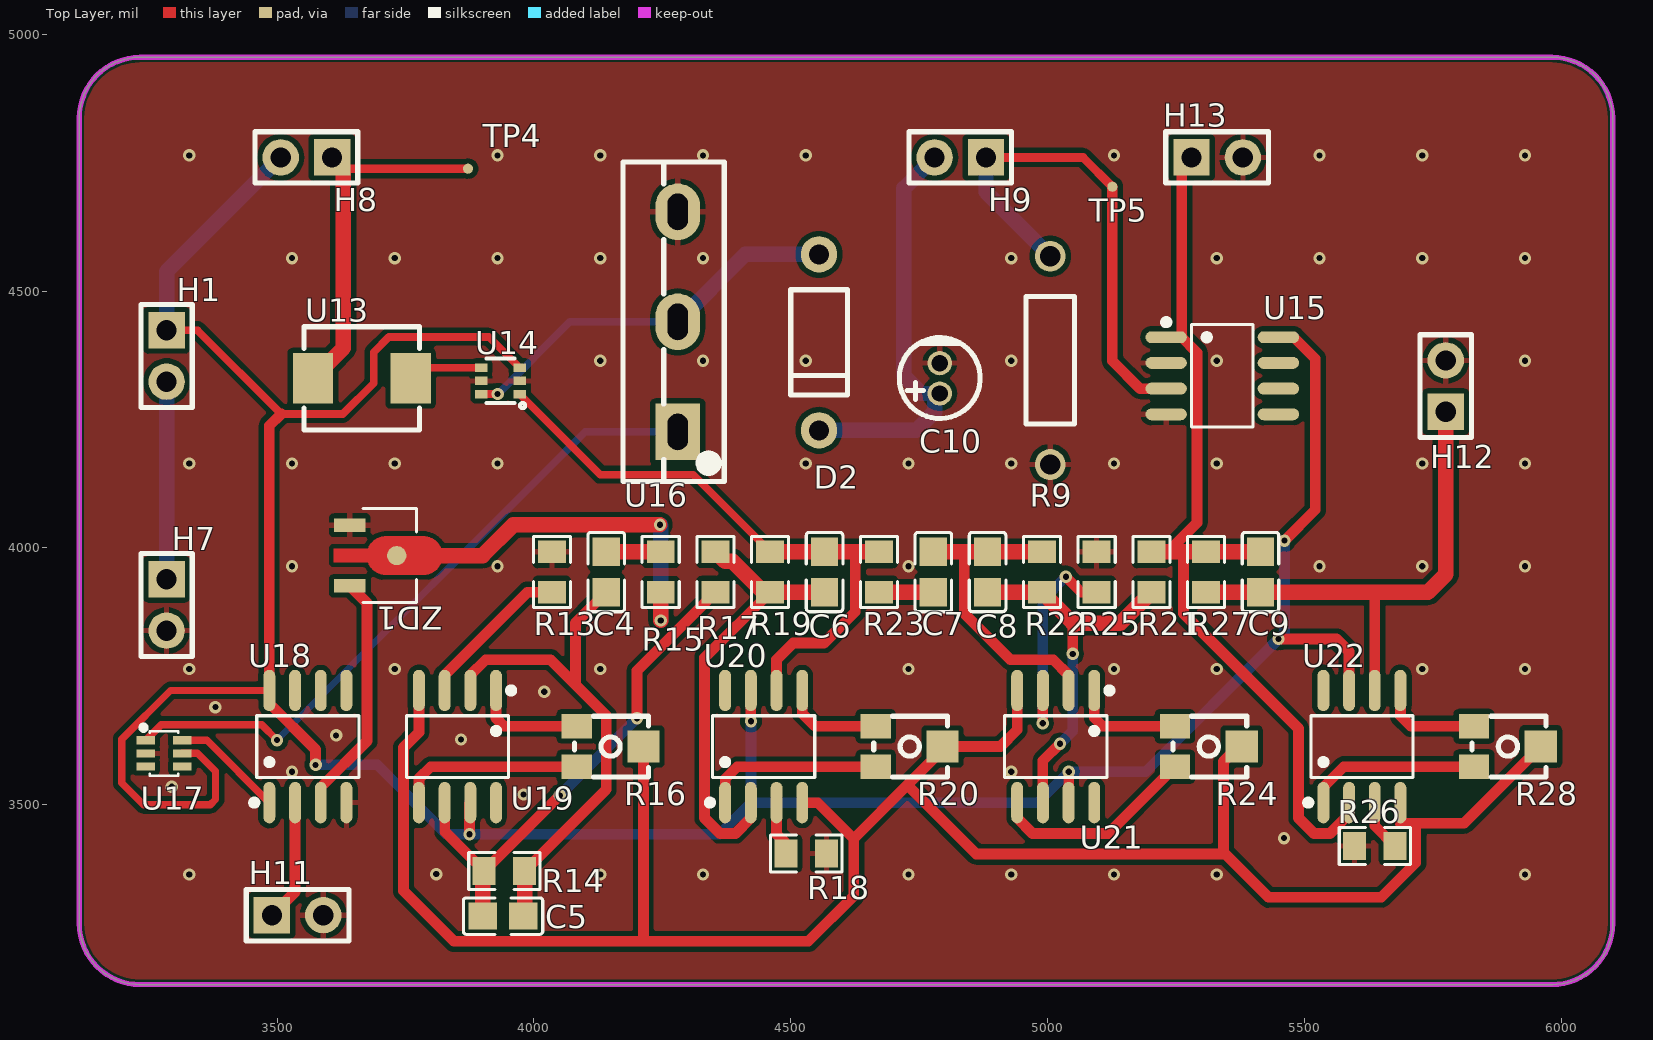
[diagram p0: Top Layer view]
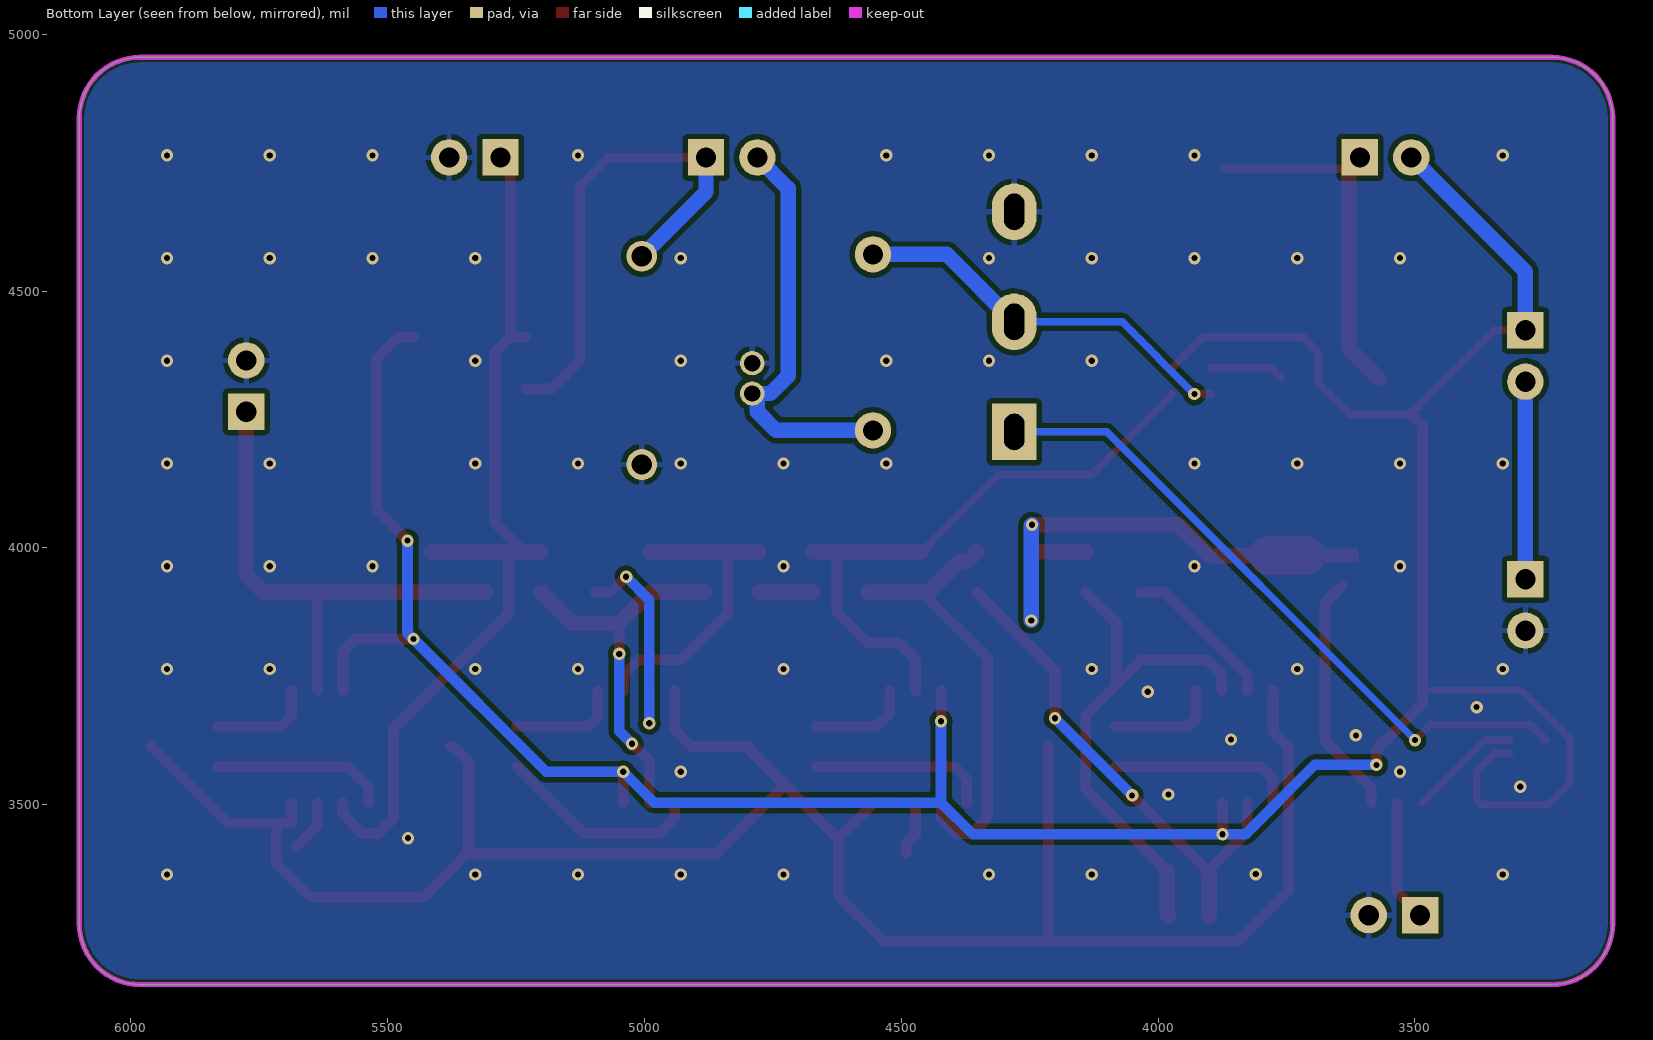
[diagram p1: Bottom Layer view, seen from below]
# Altium PCB MISC52076.pcbdoc
Units mil, origin at the board's own origin, x right, y up, seen from the top; angles counter-clockwise.
Board outline 2985 x 1805 mil, 2 copper layers (Top Layer, Bottom Layer), stack 62.206 mil thick; 45 components, 36 nets, 138 pads, 84 vias.

## Layer stack, top to bottom
Top Solder Mask Layer: solder mask 0.394, Dk 3.3
Top Layer: signal copper 1.379
Dielectric1: surface 59.449, FR4, Dk 4.5
Bottom Layer: signal copper 1.378
Bottom Solder Mask Layer: solder mask 0.394, Dk 3.3

## Board outline
3233.11,4955 ccw(c3233.11,4836.89) 3115,4836.89 3115,3268.11 ccw(c3233.11,3268.11) 3233.11,3150 5981.89,3150 ccw(c5981.89,3268.11) 6100,3268.11 6100,4836.89 ccw(c5981.89,4836.89) 5981.89,4955

## Design rules (kind name [scope] priority, off if disabled: settings)
BoardOutlineClearance copperThickness2oz_1 [All] p2 off: genericclearance=7.99 ignorepadtopadclearanceinfootprint=FALSE except(0: Arc-SplitContinuation Track-SplitContinuation SMDPad-SplitContinuation THPad-SplitContinuation Via-SplitContinuation Fill-SplitContinuation Region-SplitContinuation Poly-SplitContinuation Text-SplitContinuation Hole-SplitContinuation; 5.98: Arc-CutoutEdge Track-CutoutEdge SMDPad-CutoutEdge THPad-CutoutEdge Via-CutoutEdge Text-CutoutEdge; 6.89: Hole-OutlineEdge Hole-CutoutEdge; 10: Poly-OutlineEdge Poly-CutoutEdge; 11.81: Arc-OutlineEdge Track-OutlineEdge SMDPad-OutlineEdge THPad-OutlineEdge Via-OutlineEdge Fill-OutlineEdge Region-OutlineEdge Text-OutlineEdge Fill-CutoutEdge Region-CutoutEdge)
BoardOutlineClearance Plane_innerPlane_1 [All] p4 off: genericclearance=4.02 ignorepadtopadclearanceinfootprint=FALSE except(0: Arc-SplitContinuation Track-SplitContinuation SMDPad-SplitContinuation THPad-SplitContinuation Via-SplitContinuation Fill-SplitContinuation Region-SplitContinuation Poly-SplitContinuation Text-SplitContinuation Hole-SplitContinuation; 5.98: Arc-CutoutEdge Track-CutoutEdge SMDPad-CutoutEdge THPad-CutoutEdge Via-CutoutEdge Text-CutoutEdge; 6.89: Hole-OutlineEdge Hole-CutoutEdge; 10: Poly-OutlineEdge Poly-CutoutEdge; 11.81: Arc-OutlineEdge Track-OutlineEdge SMDPad-OutlineEdge THPad-OutlineEdge Via-OutlineEdge Fill-OutlineEdge Region-OutlineEdge Text-OutlineEdge Fill-CutoutEdge Region-CutoutEdge)
BoardOutlineClearance Copper_copperRegion_1 [All] p6 off: genericclearance=4.02 ignorepadtopadclearanceinfootprint=FALSE except(0: Arc-SplitContinuation Track-SplitContinuation SMDPad-SplitContinuation THPad-SplitContinuation Via-SplitContinuation Fill-SplitContinuation Region-SplitContinuation Poly-SplitContinuation Text-SplitContinuation Hole-SplitContinuation; 5.98: Arc-CutoutEdge Track-CutoutEdge SMDPad-CutoutEdge THPad-CutoutEdge Via-CutoutEdge Text-CutoutEdge; 6.89: Hole-OutlineEdge Hole-CutoutEdge; 10: Poly-OutlineEdge Poly-CutoutEdge; 11.81: Arc-OutlineEdge Track-OutlineEdge SMDPad-OutlineEdge THPad-OutlineEdge Via-OutlineEdge Fill-OutlineEdge Region-OutlineEdge Text-OutlineEdge Fill-CutoutEdge Region-CutoutEdge)
BoardOutlineClearance copperThickness1oz_1 [All] p8: genericclearance=4.02 ignorepadtopadclearanceinfootprint=FALSE except(0: Arc-SplitContinuation Track-SplitContinuation SMDPad-SplitContinuation THPad-SplitContinuation Via-SplitContinuation Fill-SplitContinuation Region-SplitContinuation Poly-SplitContinuation Text-SplitContinuation Hole-SplitContinuation; 5.98: Arc-CutoutEdge Track-CutoutEdge SMDPad-CutoutEdge THPad-CutoutEdge Via-CutoutEdge Text-CutoutEdge; 6.89: Hole-OutlineEdge Hole-CutoutEdge; 10: Poly-OutlineEdge Poly-CutoutEdge; 11.81: Arc-OutlineEdge Track-OutlineEdge SMDPad-OutlineEdge THPad-OutlineEdge Via-OutlineEdge Fill-OutlineEdge Region-OutlineEdge Text-OutlineEdge Fill-CutoutEdge Region-CutoutEdge)
Clearance copperThickness2oz [All] p1 off: gap=7.99 ignorepadtopadclearanceinfootprint=FALSE except(5.98: SMDPad-Track SMDPad-SMDPad THPad-Track SMDPad-THPad THPad-THPad Track-Via SMDPad-Via THPad-Via Via-Via Fill-SMDPad Region-SMDPad Fill-THPad Region-THPad Fill-Via Region-Via Fill-Fill Fill-Region Region-Region Arc-Track Arc-SMDPad Arc-THPad Arc-Via Fill-Arc Region-Arc Arc-Arc Text-Track SMDPad-Text Text-THPad Text-Via Fill-Text Region-Text Arc-Text Text-Text; 6.89: Hole-Track Hole-SMDPad Hole-THPad Hole-Via Fill-Hole Region-Hole Hole-Arc Hole-Text; 10: Poly-Track Poly-SMDPad Poly-THPad Poly-Via Poly-Fill Poly-Region Poly-Poly Poly-Arc Poly-Text Poly-Hole; 11.81: Fill-Track Region-Track)
Clearance Plane_innerPlane [All] p3 off: gap=4.02 ignorepadtopadclearanceinfootprint=FALSE except(5.98: SMDPad-Track SMDPad-SMDPad THPad-Track SMDPad-THPad THPad-THPad Track-Via SMDPad-Via THPad-Via Via-Via Fill-SMDPad Region-SMDPad Fill-THPad Region-THPad Fill-Via Region-Via Fill-Fill Fill-Region Region-Region Arc-Track Arc-SMDPad Arc-THPad Arc-Via Fill-Arc Region-Arc Arc-Arc Text-Track SMDPad-Text Text-THPad Text-Via Fill-Text Region-Text Arc-Text Text-Text; 6.89: Hole-Track Hole-SMDPad Hole-THPad Hole-Via Fill-Hole Region-Hole Hole-Arc Hole-Text; 10: Poly-Track Poly-SMDPad Poly-THPad Poly-Via Poly-Fill Poly-Region Poly-Poly Poly-Arc Poly-Text Poly-Hole; 11.81: Fill-Track Region-Track)
Clearance Copper_copperRegion [All] p5 off: gap=4.02 ignorepadtopadclearanceinfootprint=FALSE except(5.98: SMDPad-Track SMDPad-SMDPad THPad-Track SMDPad-THPad THPad-THPad Track-Via SMDPad-Via THPad-Via Via-Via Fill-SMDPad Region-SMDPad Fill-THPad Region-THPad Fill-Via Region-Via Fill-Fill Fill-Region Region-Region Arc-Track Arc-SMDPad Arc-THPad Arc-Via Fill-Arc Region-Arc Arc-Arc Text-Track SMDPad-Text Text-THPad Text-Via Fill-Text Region-Text Arc-Text Text-Text; 6.89: Hole-Track Hole-SMDPad Hole-THPad Hole-Via Fill-Hole Region-Hole Hole-Arc Hole-Text; 10: Poly-Track Poly-SMDPad Poly-THPad Poly-Via Poly-Fill Poly-Region Poly-Poly Poly-Arc Poly-Text Poly-Hole; 11.81: Fill-Track Region-Track)
Clearance copperThickness1oz [All] p7: gap=4.02 ignorepadtopadclearanceinfootprint=FALSE except(5.98: SMDPad-Track SMDPad-SMDPad THPad-Track SMDPad-THPad THPad-THPad Track-Via SMDPad-Via THPad-Via Via-Via Fill-SMDPad Region-SMDPad Fill-THPad Region-THPad Fill-Via Region-Via Fill-Fill Fill-Region Region-Region Arc-Track Arc-SMDPad Arc-THPad Arc-Via Fill-Arc Region-Arc Arc-Arc Text-Track SMDPad-Text Text-THPad Text-Via Fill-Text Region-Text Arc-Text Text-Text; 6.89: Hole-Track Hole-SMDPad Hole-THPad Hole-Via Fill-Hole Region-Hole Hole-Arc Hole-Text; 10: Poly-Track Poly-SMDPad Poly-THPad Poly-Via Poly-Fill Poly-Region Poly-Poly Poly-Arc Poly-Text Poly-Hole; 11.81: Fill-Track Region-Track)
DiffPairsRouting differentialPair [All] p1: maxlimit=6 minlimit=6 mostfreqgap=6 toplayer_minwidth=5 toplayer_prefwidth=10 toplayer_maxwidth=100 toplayer_mingap=6 toplayer_prefgap=6 toplayer_maxgap=6 bottomlayer_minwidth=5 bottomlayer_prefwidth=10 bottomlayer_maxwidth=100 bottomlayer_mingap=6 bottomlayer_prefgap=6 bottomlayer_maxgap=6 maxuncoupledlength=10
HoleToHoleClearance otherClearance [All] p1: gap=11.81 allowstackedmicrovias=TRUE
Length netLength [All] p1: minlimit=0 maxlimit=0
PasteMaskExpansion pasteMaskExpansion [All] p1: expansion=0
PlaneConnect innerPlane [All] p1: planeconnectstyle=Relief reliefexpansion=20 reliefentries=4 reliefconductorwidth=10 reliefairgap=10
PolygonConnect copperRegion [All] p1: connectstyle=Relief reliefconductorwidth=10 reliefentries=4 polygonreliefangle="90 Angle" airgapwidth=10 via.connectstyle=Relief via.reliefconductorwidth=10 via.reliefentries=4 via.polygonreliefangle="90 Angle" via.airgapwidth=10
RoutingVias viaSize [All] p1: holewidth=12.01 width=24.02 viastyle="Through Hole" minholewidth=11.81 minwidth=19.68 maxholewidth=248.03 maxwidth=393.7
SolderMaskExpansion solderMaskExpansion [IsVia] p1: expansion=-1000 istentingtop=TRUE
SolderMaskExpansion solderMaskExpansion [All] p2: expansion=2.01 istentingtop=FALSE
Width copperThickness2oz_2 [All] p1 off: maxlimit=100 minlimit=8 preferedwidth=10
Width copperThickness1oz_2 [All] p2: maxlimit=100 minlimit=5 preferedwidth=30

## Components (designator, comment, footprint, x,y, rotation, side; value= is the part's Value field where it differs from the comment)
C4 "100nF" C0805 4140.89,3953.03 r270 top
C5 "1nF" C0805 3939.95,3283.27 r180 top
C6 "100nF" C0805 4565.73,3953.03 r90 top
C7 "100nF" C0805 4777.61,3953.03 r90 top
C8 "1nF" C0805 4883.03,3953.03 r270 top
C9 "100nF" C0805 5414.34,3953.03 r270 top
C10 "10uF" CAP-TH_BD4.0-P1.50-D0.8-FD 4790,4330 r90 top
D2 "" DO_1N4007 4555,4400 r90 top
H1 "" HDR-TH_2P-P2.54-V-M-1 3285,4373.54 r270 top
H7 "" HDR-TH_2P-P2.54-V-M-1 3285,3888.86 r270 top
H8 "" HDR-TH_2P-P2.54-V-M-1 3557.14,4760 r180 top
H9 "" HDR-TH_2P-P2.54-V-M-1 4830,4760 r180 top
H11 "" HDR-TH_2P-P2.54-V-M-1 3540,3285 r0 top
H12 "" HDR-TH_2P-P2.54-V-M-1 5775,4315 r90 top
H13 "" HDR-TH_2P-P2.54-V-M-1 5330,4760 r0 top
R9 "40" Res_1/4W 5005,4365 r90 top
R13 "10kΩ" R0805 4034.95,3953.03 r270 top
R14 "10kΩ" R0805 3942.53,3370.87 r180 top
R15 "100Ω" R0805 4246.84,3953.03 r90 top
R16 "100kΩ" RES-ADJ-SMD_VG039NCH 4148.25,3613.27 r180 top
R17 "10kΩ" R0805 4353.31,3953.03 r90 top
R18 "10kΩ" R0805 4530,3405 r180 top
R19 "1MΩ" R0805 4459.78,3953.03 r90 top
R20 "100kΩ" RES-ADJ-SMD_VG039NCH 4730.5,3613.27 r180 top
R21 "10kΩ" R0805 5095.44,3953.03 r270 top
R22 "10kΩ" R0805 4988.97,3953.03 r270 top
R23 "100Ω" R0805 4671.67,3953.03 r270 top
R24 "100kΩ" RES-ADJ-SMD_VG039NCH 5312.75,3613.27 r180 top
R25 "10kΩ" R0805 5201.92,3953.03 r90 top
R26 "10kΩ" R0805 5636.95,3419.5 r0 top
R27 "1MΩ" R0805 5308.39,3953.03 r270 top
R28 "100kΩ" RES-ADJ-SMD_VG039NCH 5895,3613.27 r180 top
TP4 "" Test-Point-0.5mm 3871.67,4738.07 r0 top
TP5 "" Test-Point-0.5mm 5125.97,4703.07 r0 top
U13 "Power inductor (SMD), CKST0502-10uH/M, 10uH, ±20%, 3A, package 5.7mm*5.1mm*2.0mm, Cenke, RoHS" IND-SMD_L5.7-W5.1 3665,4330 r0 top
U14 "INA199A3DCKT" SC-70-6_L2.1-W1.3-P0.65-LS2.1-BR 3935,4325 r0 top
U15 "NE5532DR" SOIC-8_L4.9-W3.9-P1.27-LS6.0-BL 5340,4335 r270 top
U16 "HY5204" TO-247-3_L15.8-W5.0-P5.44-L-1 4280,4440 r90 top
U17 "SN74LVC2G04DCKR" SOT-363_L2.0-W1.3-P0.65-LS2.1-BR 3280,3600 r180 top
U18 "NE5532DR" SOIC-8_L4.9-W3.9-P1.27-LS6.0-BL 3560,3613.27 r0 top
U19 "UA741CDT" SOIC-8_L4.9-W3.9-P1.27-LS6.0-BL 3851.24,3613.27 r180 top
U20 "UA741CDT" SOIC-8_L4.9-W3.9-P1.27-LS6.0-BL 4447.23,3613.27 r0 top
U21 "UA741CDT" SOIC-8_L4.9-W3.9-P1.27-LS6.0-BL 5015.74,3613.27 r180 top
U22 "UA741CDT" SOIC-8_L4.9-W3.9-P1.27-LS6.0-BL 5611.73,3613.27 r0 top
ZD1 "" SOT-89-3_L4.5-W2.5-P1.50-LS4.2-BR 3695,3985 r180 top

## Footprints (in the part's own frame and the unit in brackets; to place one, negate y for a bottom-side part, rotate by r counter-clockwise, add the part's x,y. Pads: shape width x height; smd on the part's side, far side on the other; paste and mask are expansions set on the pad)
C0805 [mm]
  rect 1.41x1.35 smd paste-100 mask+0.051: 1(-1,0) 2(1,0)
  silkscreen extent -1.96,-0.9 1.96,0.9
CAP-TH_BD4.0-P1.50-D0.8-FD [mm]
  round 1.2 hole 0.8: 1(-0.75,0) 2(0.75,0)
  silkscreen extent -1.98,-2 2.06,2
DO_1N4007 [mm]
  round 1.8 hole 1 paste+0 mask+0.051: 1(-4.35,0) 2(4.35,0)
  silkscreen extent -2.6,-1.4 2.6,1.4
HDR-TH_2P-P2.54-V-M-1 [mm]
  rect 1.8x1.8 hole 1: 1(-1.27,0)
  round 1.8 hole 1: 2(1.27,0)
  silkscreen extent -2.54,-1.27 2.54,1.27
IND-SMD_L5.7-W5.1 [mm]
  rect 2x2.5 smd paste+0 mask+0.05: 1(-2.413,0) 2(2.413,0)
  silkscreen extent -2.85,-2.55 2.85,2.55
R0805 [mm]
  rect 1.133x1.377 smd paste-100 mask+0.051: 1(-1,0) 2(1,0)
  silkscreen extent -1.76,-0.92 1.76,0.92
RES-ADJ-SMD_VG039NCH [mm]
  rect 1.5x1.2 smd: 1(1.65,-1) 3(1.65,1)
  rect 1.6x1.6 smd: 2(-1.65,0)
  silkscreen extent -1.9,-1.5 1.75,1.5
Res_1/4W [mil]
  round 60 hole 39.37 paste+0 mask+2: 1(-202.76,0) 2(202.76,0)
  silkscreen extent -124,-47 124,47
SC-70-6_L2.1-W1.3-P0.65-LS2.1-BR [mm]
  rect 0.6x0.42 smd: 1(0.95,-0.65) 2(0.95,0) 3(0.95,0.65) 4(-0.95,0.65) 5(-0.95,0) 6(-0.95,-0.65)
  silkscreen extent -0.7,-1.34 1.22,1.1
SOIC-8_L4.9-W3.9-P1.27-LS6.0-BL [mm]
  oval 0.588x2.045 smd: 1(-1.905,-2.772) 2(-0.635,-2.772) 3(0.635,-2.772) 4(1.905,-2.772) 5(1.905,2.772) 6(0.635,2.772) 7(-0.635,2.772) 8(-1.905,2.772)
  silkscreen extent -2.8,-2.92 2.53,1.52
SOT-89-3_L4.5-W2.5-P1.50-LS4.2-BR [mm]
  rect 1.575x0.672 smd: 1(1.356,-1.5) 3(1.356,1.5)
  round 0.95 smd: 2(-0.966,0)
  Top Layer region: -2.283,0.95 -0.429,0.95 -0.384,0.949 -0.34,0.946 -0.296,0.94 -0.252,0.933 -0.208,0.924 -0.165,0.912 -0.123,0.899 -0.081,0.884 -0.04,0.866 0,0.847 0.04,0.826 0.078,0.803 0.115,0.779 0.151,0.752 0.185,0.724 0.219,0.695 0.251,0.664 0.281,0.631 0.31,0.597 0.337,0.562 0.362,0.525 0.386,0.488 0.408,0.449 0.428,0.409 0.447,0.33 2.144,0.33 2.144,-0.33 0.447,-0.33 0.428,-0.409 0.408,-0.449 0.386,-0.488 0.362,-0.526 0.337,-0.562 0.31,-0.597 0.281,-0.631 0.251,-0.664 0.219,-0.695 0.185,-0.725 0.151,-0.753 0.115,-0.779 0.078,-0.804 0.04,-0.827 0,-0.848 -0.04,-0.867 -0.081,-0.884 -0.123,-0.899 -0.165,-0.913 -0.208,-0.924 -0.252,-0.934 -0.296,-0.941 -0.34,-0.946 -0.384,-0.949 -0.429,-0.95 -2.283,-0.95 -2.328,-0.949 -2.372,-0.946 -2.416,-0.941 -2.46,-0.934 -2.504,-0.924 -2.547,-0.913 -2.589,-0.899 -2.631,-0.884 -2.672,-0.867 -2.713,-0.848 -2.752,-0.827 -2.79,-0.804 -2.827,-0.779 -2.863,-0.753 -2.898,-0.725 -2.931,-0.695 -2.963,-0.664 -2.993,-0.631 -3.022,-0.597 -3.049,-0.562 -3.075,-0.526 -3.098,-0.488 -3.12,-0.449 -3.141,-0.409 -3.159,-0.369 -3.175,-0.327 -3.189,-0.285 -3.202,-0.242 -3.212,-0.199 -3.22,-0.155 -3.227,-0.111 -3.231,-0.067 -3.233,-0.022 -3.233,0.022 -3.231,0.067 -3.227,0.111 -3.22,0.155 -3.212,0.199 -3.202,0.242 -3.189,0.285 -3.175,0.327 -3.159,0.369 -3.141,0.409 -3.12,0.449 -3.098,0.488 -3.075,0.525 -3.049,0.562 -3.022,0.597 -2.993,0.631 -2.963,0.664 -2.931,0.695 -2.898,0.724 -2.863,0.752 -2.827,0.779 -2.79,0.803 -2.752,0.826 -2.713,0.847 -2.672,0.866 -2.631,0.884 -2.589,0.899 -2.547,0.912 -2.504,0.924 -2.46,0.933 -2.416,0.94 -2.372,0.946 -2.328,0.949
  silkscreen extent -1.95,-2.33 0.7,2.33
SOT-363_L2.0-W1.3-P0.65-LS2.1-BR [mm]
  rect 0.9x0.4 smd: 1(0.9,-0.65) 2(0.9,0) 3(0.9,0.65) 4(-0.9,0.65) 5(-0.9,0) 6(-0.9,-0.65)
  silkscreen extent -0.7,-1.4 1.14,1.1
Test-Point-0.5mm [mm]
  round 0.5 smd: 1(0,0)
TO-247-3_L15.8-W5.0-P5.44-L-1 [mm]
  rect 2.8x2.2 hole 1 slot 1.8 at 0 deg paste+0 mask+0.05: 1(-5.44,0)
  oval 2.8x2.2 hole 1 slot 1.8 at 0 deg paste+0 mask+0.05: 2(0,0) 3(5.44,0)
  silkscreen extent -7.9,-2.3 7.9,2.7

## Via types
v1: diameter 24.02, hole 12, Top Layer to Bottom Layer, 84 vias

## Nets (pads, with @x,y where several pads share a name; then routed paths per layer and width w, separated by ;. In a path a pad name is that pad's centre, name@x,y a point inside that pad or via, vN(x,y) a via of type N, cw(c..) or ccw(c..) an arc to the next point about the centre after c; other vN are vias at no path point)
$1N5592: H8.1 TP4.1 U13.1 | length 706.1
  Top Layer w16.84: H8.1 3629.07,4738.07 TP4.1
  Top Layer w30: U13.1 3629.07,4389.07 H8.1@3629.07,4738.07
$1N5597: H1.2 H7.1 | length 384.7
  Bottom Layer w30: H7.1 H1.2
$1N5640: U13.2 U14.4 | length 146.1
  Top Layer w14.88: U13.2 3780.59,4350.59 U14.4
$1N5681: D2.2 U14.6 U16.2 | length 770
  Top Layer w14.88: U14.6 v1(3929.41,4299.41)
  Bottom Layer w14.88: v1(3929.41,4299.41) 4070,4440 U16.2
  Bottom Layer w30: U16.2 4411.26,4571.26 D2.2
$1N5747: C10.1 D2.1 H9.2 | length 809.6
  Bottom Layer w30: D2.1 4743.74,4228.74 4780,4265 C10.1@4780,4300.47 ; H9.2 4720,4700 4720,4335 4754.53,4300.47 C10.1@4780,4300.47 ; C10.1 C10.1@4780,4300.47
$1N5786: H9.1 R9.2 TP5.1 U15.3 | length 979.9
  Top Layer w16.84: H9.1 5069.04,4760 TP5.1
  Top Layer w20.84: TP5.1 5125.97,4364.03 5180,4310 U15.3
  Bottom Layer w30: H9.1 4880,4692.76 R9.2
$1N6149: U16.1 U17.1 | length 1308.9
  Top Layer w14.17: U17.1 3274.82,3655.83 3470,3655.83 v1(3500,3625.83)
  Bottom Layer w14.17: v1(3500,3625.83) 4100,4225.83 U16.1
$1N6347: H11.1 U18.2 | length 237.8
  Top Layer w20.84: H11.1 3535,3330 U18.2
$1N6525: U18.3 ZD1.3 | length 472.9
  Top Layer w20.84: U18.3 3585,3534.12 3675,3624.12 3675,3892.55 ZD1.3
$1N6528: R15.1 ZD1.2 | length 763.9
  Top Layer w30: ZD1.2@3748.39,3985.01 3900.01,3985.01 3960.01,4045.01 v1(4245.49,4045.01) ; v1(4246.84,3858.66) R15.1
  Bottom Layer w30: v1(4245.49,4045.01) 4246.84,4043.66 v1(4246.84,3858.66)
$1N6877: C5.2 R14.2 R17.1 U19.6 | length 983
  Top Layer w20.84: U19.6 3826.24,3447.79 R14.2 v1(4050.58,3518.29) ; v1(4200.58,3668.29) 4200.58,3760.93 R17.1
  Top Layer w30: C5.2 3900.58,3368.29 R14.2
  Bottom Layer w20.84: v1(4050.58,3518.29) v1(4200.58,3668.29)
$1N6878: C4.1 R15.2 | length 105.9
  Top Layer w30: C4.1 R15.2
$1N6879: R13.2 U19.3 | length 305.5
  Top Layer w20.84: U19.3 3826.24,3752.42 3987.48,3913.66 R13.2
$1N6880: R16.1 U19.1 | length 217.4
  Top Layer w20.84: U19.1 3926.24,3668.76 3942.36,3652.64 R16.1
$1N6882: R16.3 U19.5 | length 363.6
  Top Layer w20.84: U19.5 3776.24,3551.24 3798.9,3573.9 R16.3
$1N6883: C4.2 C5.1 R14.1 U19.2 | length 1014.3
  Top Layer w20.84: U19.2 3876.24,3752.42 3906.24,3782.42 4032.13,3782.42 4080.89,3733.66 ; R14.1 4140.89,3529.86 4140.89,3673.66 4080.89,3733.66 ; C4.2 4080.89,3853.66 4080.89,3733.66
  Top Layer w30: C5.1 3981.9,3285.85 R14.1
$1N7186: R20.3 U20.1 | length 349.4
  Top Layer w20.84: U20.1 4372.23,3550.59 4395.54,3573.9 R20.3
$1N7187: R20.1 U20.5 | length 198.4
  Top Layer w20.84: U20.5 4522.23,3677.77 4547.36,3652.64 R20.1
$1N7188: R18.2 U20.3 | length 106.7
  Top Layer w20.84: U20.3 4472.23,3442.77 4490.63,3424.37 R18.2
$1N7189: C6.1 R17.2 R19.1 U20.2 | length 882.3
  Top Layer w20.84: U20.2 4422.23,3474.12 4392.23,3444.12 4362.23,3444.12 4332.23,3474.12 4332.23,3786.11 R19.1
  Top Layer w30: R17.2 4372.05,3973.66 4387.05,3973.66 4447.05,3913.66 R19.1 C6.1
$1N7811: C8.2 R22.2 R25.1 U21.6 | length 742.3
  Top Layer w20.84: U21.6 4990.74,3585.43 v1(5023.97,3618.66) ; v1(5048.97,3793.66) 5048.97,3853.66
  Top Layer w30: C8.2 R22.2 5048.97,3853.66 5141.92,3853.66 R25.1
  Bottom Layer w20.84: v1(5023.97,3618.66) 5048.97,3643.66 v1(5048.97,3793.66)
$1N7823: C7.1 R23.2 | length 105.9
  Top Layer w30: R23.2 C7.1
$1N7824: R21.2 U21.3 | length 439.9
  Top Layer w20.84: v1(4990.44,3658.66) 4990.74,3658.95 U21.3 ; v1(5035.44,3943.66) 5065.44,3913.66 R21.2
  Bottom Layer w20.84: v1(4990.44,3658.66) 4990.44,3898.66 v1(5035.44,3943.66)
$1N7825: R24.1 U21.1 | length 217.1
  Top Layer w20.84: U21.1 5090.74,3669.26 5107.36,3652.64 R24.1
$1N7827: R24.3 U21.5 | length 403.2
  Top Layer w20.84: U21.5 4940.74,3474.12 4970.74,3444.12 5118.01,3444.12 R24.3
$1N7828: C7.2 C8.1 R22.1 U21.2 | length 614.2
  Top Layer w20.84: 4837.61,3992.4 4837.61,3872.4 4927.61,3782.4 5010.75,3782.4 5040.75,3752.4 U21.2
  Top Layer w30: C7.2 4837.61,3992.4 C8.1 R22.1
$1N7831: R28.3 U22.1 | length 339.8
  Top Layer w20.84: U22.1 5536.73,3534.12 5576.52,3573.9 R28.3
$1N7832: R28.1 U22.5 | length 201
  Top Layer w20.84: U22.5 5686.73,3673.27 5707.36,3652.64 R28.1
$1N7833: R26.2 U22.3 | length 101
  Top Layer w20.84: U22.3 5636.73,3459.09 R26.2
$1N7837: C9.2 H12.1 R27.2 U22.6 | length 988.9
  Top Layer w20.84: U22.6 5636.73,3913.66
  Top Layer w30: R27.2 C9.2 5636.73,3913.66 5740.39,3913.66 5775,3948.27 H12.1
-VCC: R16.2 R20.2 R24.2 R28.2 U19.4 U20.4 U21.4 U22.4 | length 4247.9
  Top Layer w20.84: U19.4 3776.24,3641.24 3746.24,3611.24 3746.24,3332.42 3844.54,3234.12 4213.21,3234.12 ; R16.2 4213.21,3234.12 ; U20.4 4552.23,3504.12 4622.36,3433.99 ; U21.4 4940.74,3645.74 4908.27,3613.27 R20.2 4795.46,3607.09 4726.69,3538.31 ; 5342.36,3403.99 4861.01,3403.99 4726.69,3538.31 ; R24.2 5371.64,3613.27 5342.36,3583.99 5342.36,3407.64 5430,3320 5649.67,3320 5716.73,3387.06 5716.73,3463.99 ; U22.4 5686.73,3463.99 5716.73,3463.99 ; R28.2 5810.68,3463.99 5716.73,3463.99 ; 4213.21,3234.12 4534.12,3234.12 4622.36,3322.36 4622.36,3433.99 ; 4622.36,3433.99 4726.69,3538.31
GND: C10.2 H7.2 H11.2 H12.2 H13.2 R9.1 R13.1 R18.1 R21.1 R26.1 U14.2 U14.5 U15.2 U15.4 U16.3 U17.2 U18.4 ZD1.1
  other v1: 3329.1,3364.1 4129.1,3364.1 4329.1,3364.1 4729.1,3364.1 4929.1,3364.1 5129.1,3364.1 5329.1,3364.1 5929.1,3364.1 3810,3365 5460,3435 3980,3520 3295,3535 3529.1,3564.1 4929.1,3564.1 3858.11,3626.94 3615,3635 3380,3690 4020,3720 3329.1,3764.1 3729.1,3764.1 4129.1,3764.1 4729.1,3764.1 5129.1,3764.1 5329.1,3764.1 5729.1,3764.1 5929.1,3764.1 3529.1,3964.1 3929.1,3964.1 4729.1,3964.1 5529.1,3964.1 5729.1,3964.1 5929.1,3964.1 3329.1,4164.1 3529.1,4164.1 3729.1,4164.1 3929.1,4164.1 4529.1,4164.1 4729.1,4164.1 4929.1,4164.1 5129.1,4164.1 5329.1,4164.1 5729.1,4164.1 5929.1,4164.1 4129.1,4364.1 4329.1,4364.1 4529.1,4364.1 4929.1,4364.1 5329.1,4364.1 5929.1,4364.1 3529.1,4564.1 3729.1,4564.1 3929.1,4564.1 4129.1,4564.1 4329.1,4564.1 4929.1,4564.1 5329.1,4564.1 5529.1,4564.1 5729.1,4564.1 5929.1,4564.1 3329.1,4764.1 3929.1,4764.1 4129.1,4764.1 4329.1,4764.1 4529.1,4764.1 5129.1,4764.1 5529.1,4764.1 5729.1,4764.1 5929.1,4764.1
IL: C6.2 R19.2 R23.1 U14.1 U20.6 | length 1195
  Top Layer w14.88: U14.1 4129.41,4142.4 4309.78,4142.4 R19.2
  Top Layer w20.84: U20.6 4472.23,3782.23 4505,3815 4564.82,3815 4625.73,3875.91 4625.73,3992.4
  Top Layer w30: R19.2 C6.2 4625.73,3992.4 R23.1
PWM: U17.6 U18.1 | length 219.9
  Top Layer w14.17: U17.6 3363.53,3625.59 U18.1
VCC: H1.1 H8.2 U14.3 U15.8 U17.5 U18.8 U19.7 U20.7 U21.7 U22.7 | length 6100.8
  Top Layer w14.17: U17.5 3345.03,3600 3380.02,3565 3380.02,3510.02 3370,3500 3240,3500 3197.86,3542.14 3197.86,3627.57 3292.7,3722.42 U18.8
  Top Layer w14.88: H1.1 3345,4423.54 3507.95,4260.59 3627.95,4260.59 3687.95,4320.59 3687.95,4380.59 3717.95,4410.59 3912.4,4410.59 U14.3
  Top Layer w20.84: 3507.95,4260.59 3485,4237.64 U18.8 3485,3697.64 3575,3607.64 v1(3575,3577.64) ; v1(3874.75,3442.64) 3874.75,3502.64 U19.7 ; U20.7 4422.23,3662.85 v1(4422.45,3662.64) ; U21.7 v1(5040.97,3564.12) ; U15.8 5479.15,4410 5520.97,4368.18 5520.97,4074.12 v1(5460.97,4014.12) ; v1(5449.38,3822.53) 5562.47,3822.53 5586.73,3798.27 U22.7
  Bottom Layer w20.84: v1(3575,3577.64) 3695,3577.64 3830,3442.64 v1(3874.75,3442.64) 4360.97,3442.64 4422.45,3504.12 ; v1(4422.45,3662.64) 4422.45,3504.12 ; v1(5460.97,4014.12) 5460.97,3834.12 v1(5449.38,3822.53) 5190.97,3564.12 v1(5040.97,3564.12) 4980.97,3504.12 4422.45,3504.12
  Bottom Layer w30: H1.1 3285,4537.86 H8.2
VO: C9.1 H13.1 R25.2 R27.1 U15.1 U22.2 | length 1813.9
  Top Layer w20.84: U15.1 U15.1@5260.85,4410 ; 5234.34,3992.4 5290.85,4048.91 5290.85,4380 U15.1@5260.85,4410 ; 5264.34,3992.4 5264.34,3872.4 5488.45,3648.29 5488.45,3474.12 5518.45,3444.12 5549.6,3444.12 5586.73,3481.25 U22.2 ; H13.1 5260.85,4740.85 U15.1@5260.85,4410
  Top Layer w30: R25.2 5234.34,3992.4 5264.34,3992.4 R27.1 C9.1
pads on no net: U15.5 U15.6 U15.7 U17.3 U17.4 U18.5 U18.6 U18.7 U19.8 U20.8 U21.8 U22.8

## Polygon pours and split planes (outlines as drawn)
GND on Top Layer (solid, remove dead copper, pour order 0): 3020,5060 3020,3000 6160,3000 6160,5060
GND on Bottom Layer (solid, remove dead copper, pour order 2): 3000,5070 3000,3005 6195,3005 6195,5070

## Keep-outs
Board Outline Layer:
  the board outline again, w10